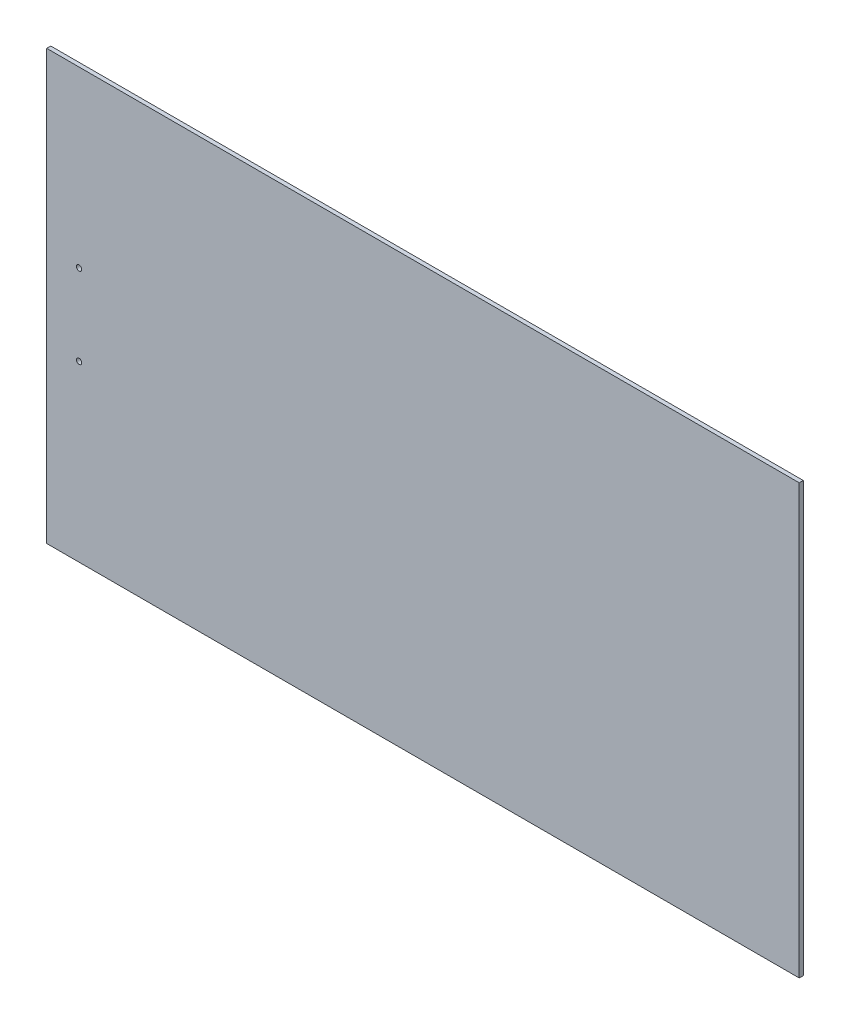
SolidWorks part; units mm, degrees
ref_plane "前视基准面" through (0, 0, 0) normal (0, 0, 1) x (1, 0, 0)
ref_plane "上视基准面" through (0, 0, 0) normal (0, 1, 0) x (1, 0, 0)
ref_plane "右视基准面" through (0, 0, 0) normal (1, 0, 0) x (0, 0, -1)
sketch "草图1" plane through (0, 0, 0) normal (0, 0, 1) x (1, 0, 0)
  line L1 (465, -265) -> (-465, -265)
  line L2 (465, -265) -> (465, 265)
  line L3 (465, 265) -> (-465, 265)
  line L4 (-465, -265) -> (-465, 265)
  line L5 (465, -265) -> (-465, 265) construction
  line L6 (465, 265) -> (-465, -265) construction
  point P0 (0, 0)
  dimension "D1" = 930
  dimension "D2" = 530
extrude "凸台-拉伸1" add sketch "草图1" along normal blind 5
sketch "草图2" plane through (0, 0, 0) normal (0, 0, -1) x (-1, 0, 0)
  line L0 (465, 0) -> (425, 0) construction
  line L1 (465, 265) -> (465, -265) construction
  line L2 (425, 50) -> (425, -50) construction
  circle A0 centre (425, 50) radius 3.3
  circle A1 centre (425, -50) radius 3.3
  dimension "D3" = 6.6
  dimension "D1" = 100
  dimension "D2" = 40
extrude "切除-拉伸1" cut sketch "草图2" against normal blind 10
